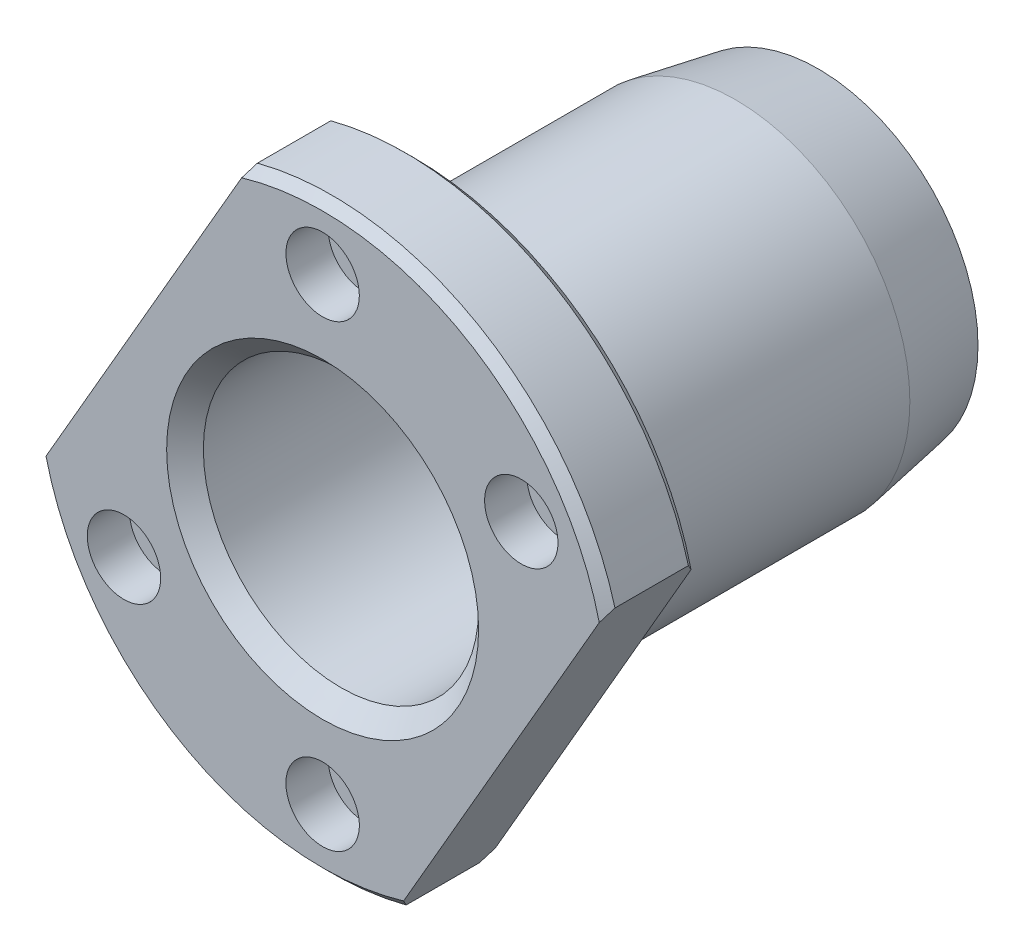
from build123d import *

# Parameters (mm, degrees)
SKETCH1_R                                            = 19
BOSS_EXTRUDE1_DEPTH                                  = 45
SKETCH2_R                                            = 15
CUT_EXTRUDE1_DEPTH                                   = 30
M18X1_5_TAPPED_HOLE1_D                               = 16.5
M18X1_5_TAPPED_HOLE1_DEPTH                           = 43.5
M18X1_5_TAPPED_HOLE1_TIP                             = 4.957100107
BOSS_EXTRUDE2_START                                  = 10
SKETCH5_R                                            = 32
SKETCH5_R_2                                          = 15
BOSS_EXTRUDE2_DEPTH                                  = 10
HOLE_SIZE_PER_SOCKET_HEAD_CAP_SCREW_TYPE_D           = 4.5
HOLE_SIZE_PER_SOCKET_HEAD_CAP_SCREW_TYPE_CBORE_D     = 8
HOLE_SIZE_PER_SOCKET_HEAD_CAP_SCREW_TYPE_CBORE_DEPTH = 4.6
CIRPATTERN1_COUNT                                    = 6
CUT_EXTRUDE2_REACH                                   = 73.225
CHAMFER1_SIZE                                        = 1
CHAMFER2_SIZE                                        = 10
CHAMFER2_SIZE2                                       = 1.763269807
CHAMFER3_SIZE                                        = 1
CHAMFER3_SIZE2                                       = 1.232803052
CHAMFER4_SIZE                                        = 2


with BuildPart() as part:
    # Sketch1 → Boss-Extrude1 (new body)
    with BuildSketch(Plane.XY):
        with Locations(Location((0, 0, 0), (0, 0, 180))):
            Circle(SKETCH1_R)
    extrude(amount=BOSS_EXTRUDE1_DEPTH)

    # Sketch2 → Cut-Extrude1 (cut)
    with BuildSketch(Plane.XY.offset(45)):
        Circle(SKETCH2_R)
    extrude(amount=-CUT_EXTRUDE1_DEPTH, mode=Mode.SUBTRACT)

    # M18x1.5 Tapped Hole1
    with Locations(Plane(origin=(0, 0, 0), x_dir=(-1, 0, 0), z_dir=(0, 0, -1))):
        with Locations((0, 0)):
            Hole(M18X1_5_TAPPED_HOLE1_D / 2, depth=M18X1_5_TAPPED_HOLE1_DEPTH)
            with Locations((0, 0, -(M18X1_5_TAPPED_HOLE1_DEPTH + M18X1_5_TAPPED_HOLE1_TIP / 2))):  # 118° drill point
                Cone(0, M18X1_5_TAPPED_HOLE1_D / 2, M18X1_5_TAPPED_HOLE1_TIP, mode=Mode.SUBTRACT)

    # Sketch5 → Boss-Extrude2 (add)
    with BuildSketch(Plane.XY.offset(45).offset(BOSS_EXTRUDE2_START)):
        Circle(SKETCH5_R)
        Circle(SKETCH5_R_2, mode=Mode.SUBTRACT)
    extrude(amount=-BOSS_EXTRUDE2_DEPTH)

    # Hole size per socket head cap screw type1 (through all)
    with Locations(Plane(origin=(0, 25, 55), x_dir=(1, 0, 0), z_dir=(0, 0, 1))):
        with Locations((0, 0)):
            hole_size_per_socket_head_cap_screw_type = CounterBoreHole(HOLE_SIZE_PER_SOCKET_HEAD_CAP_SCREW_TYPE_D / 2, HOLE_SIZE_PER_SOCKET_HEAD_CAP_SCREW_TYPE_CBORE_D / 2, HOLE_SIZE_PER_SOCKET_HEAD_CAP_SCREW_TYPE_CBORE_DEPTH)

    # CirPattern1: Hole size per socket head cap screw type1 ×6 about axis, 2 skipped
    cirpattern1_axis = Axis((0, 0, 55), (0, 0, 1))
    add([hole_size_per_socket_head_cap_screw_type.rotate(cirpattern1_axis, i * 360 / CIRPATTERN1_COUNT) for i in range(1, CIRPATTERN1_COUNT) if i not in (1, 4)], mode=Mode.SUBTRACT)

    # Sketch7 → Cut-Extrude2 (cut, up to next)
    with BuildSketch(Plane.XY.offset(55), mode=Mode.PRIVATE) as cut_extrude2_sk1:
        with BuildLine():
            Line((-8.108511332, 30.955646399), (-30.862631838, -8.455646399))
            ThreePointArc((-30.862631838, -8.455646399), (-27.712812921, 16), (-8.108511332, 30.955646399))
        make_face()
    cut_extrude2_tool1 = extrude(cut_extrude2_sk1.sketch, amount=-CUT_EXTRUDE2_REACH, mode=Mode.PRIVATE) & part.part
    # Sketch7 → Cut-Extrude2 (cut, up to next)
    with BuildSketch(Plane.XY.offset(55), mode=Mode.PRIVATE) as cut_extrude2_sk2:
        with BuildLine():
            Line((30.862631838, 8.455646399), (8.108511332, -30.955646399))
            ThreePointArc((8.108511332, -30.955646399), (27.712812921, -16), (30.862631838, 8.455646399))
        make_face()
    cut_extrude2_tool2 = extrude(cut_extrude2_sk2.sketch, amount=-CUT_EXTRUDE2_REACH, mode=Mode.PRIVATE) & part.part
    add(cut_extrude2_tool1.solids().sort_by_distance((-22.822298, 13.17646, 55))[0], mode=Mode.SUBTRACT)
    add(cut_extrude2_tool2.solids().sort_by_distance((22.822298, -13.17646, 55))[0], mode=Mode.SUBTRACT)

    # Chamfer1
    chamfer1_edges = [part.edges().sort_by_distance(p)[0] for p in [
        (-16, -27.712812921, 55),
        (-16, -27.712812921, 45),
        (16, 27.712812921, 55),
        (16, 27.712812921, 45),
    ]]
    chamfer(chamfer1_edges, length=CHAMFER1_SIZE)

    # Chamfer2
    chamfer2_edges = [part.edges().sort_by_distance(p)[0] for p in [
        (19, 0, 0),
    ]]
    chamfer2_side = [part.faces().sort_by_distance(p)[0] for p in [
        (19, 0, 22.5),
    ]]
    chamfer(chamfer2_edges, length=CHAMFER2_SIZE, length2=CHAMFER2_SIZE2, reference=chamfer2_side[0])

    # Chamfer3
    chamfer3_edges = [part.edges().sort_by_distance(p)[0] for p in [
        (17.236730193, 0, 0),
    ]]
    chamfer3_side = [part.faces().sort_by_distance(p)[0] for p in [
        (18.118365096, 0, 5),
    ]]
    chamfer(chamfer3_edges, length=CHAMFER3_SIZE, length2=CHAMFER3_SIZE2, reference=chamfer3_side[0])

    # Chamfer4
    chamfer4_edges = [part.edges().sort_by_distance(p)[0] for p in [
        (-15, 0, 55),
    ]]
    chamfer(chamfer4_edges, length=CHAMFER4_SIZE)


solid = part.part
